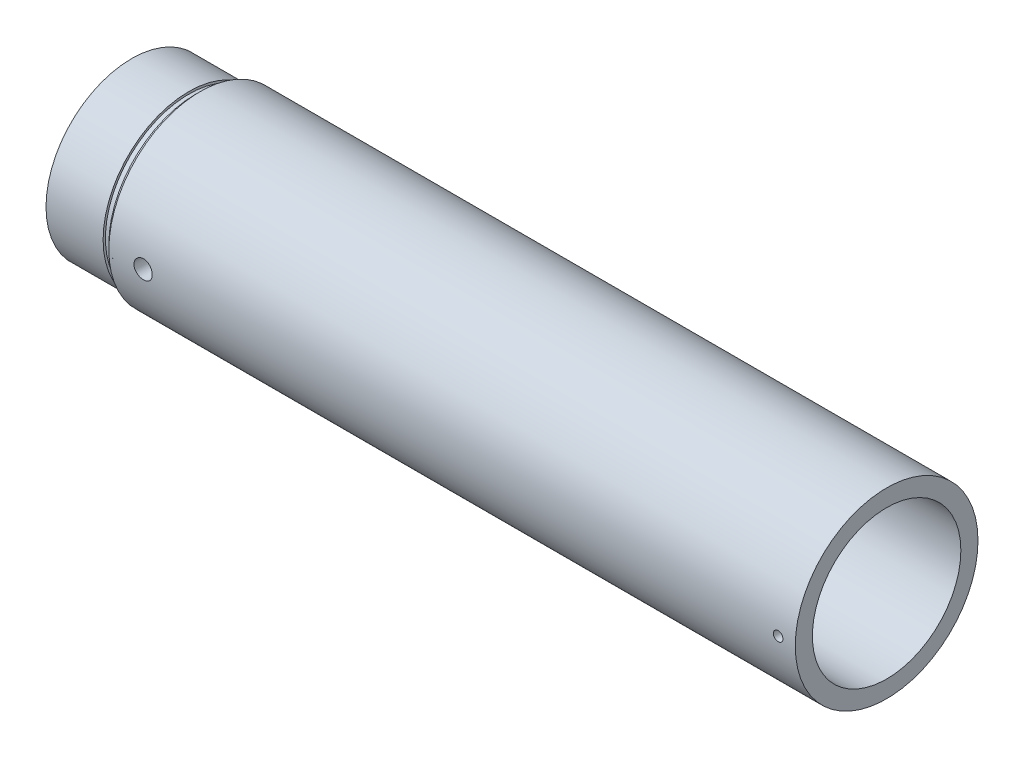
SolidWorks part; units mm, degrees
ref_plane "Front Plane" through (0, 0, 0) normal (0, 0, 1) x (1, 0, 0)
ref_plane "Top Plane" through (0, 0, 0) normal (0, 1, 0) x (1, 0, 0)
ref_plane "Right Plane" through (0, 0, 0) normal (1, 0, 0) x (0, 0, -1)
sketch "Sketch1" plane through (0, 0, 0) normal (0, 0, 1) x (1, 0, 0)
  line L0 (0, 0) -> (-259.6447, 0) construction
  line L1 (0, 0) -> (0, 37.5)
  line L2 (0, 37.5) -> (25, 37.5)
  line L3 (25, 37.5) -> (25, 36.5)
  line L4 (25, 36.5) -> (28, 36.5)
  line L5 (28, 36.5) -> (28, 38)
  line L6 (28, 38) -> (30, 38)
  line L7 (30, 38) -> (30, 40)
  line L8 (30, 40) -> (330.5, 40)
  line L9 (330.5, 40) -> (330.5, 0)
  line L10 (330.5, 0) -> (0, 0)
  dimension "D1" = 37.5
  dimension "D2" = 38
  dimension "D3" = 36.5
  dimension "D4" = 3
  dimension "D5" = 25
  dimension "D6" = 30
  dimension "D7" = 40
  dimension "D8" = 330.5
revolve "Revolve1" add sketch "Sketch1" angle 360 about L0
sketch "Sketch2" plane through (330.5, 0, 0) normal (1, 0, 0) x (0, 0, -1)
  circle A0 centre (0, 0) radius 32.5
  dimension "D1" = 65
extrude "Cut-Extrude1" cut sketch "Sketch2" against normal blind 50
cosmetic thread "Cosmetic Thread2" parameters "D2"=66
sketch "Sketch3" plane through (280.5, 0, 0) normal (1, 0, 0) x (0, 0, -1)
  circle A0 centre (0, 0) radius 30
  dimension "D1" = 60
extrude "Cut-Extrude2" cut sketch "Sketch3" against normal through all
chamfer "Chamfer1" distance 1.5 angle 45 1 edges at (280.5, 0, -32.5)
chamfer "Chamfer2" distance 1.5 angle 45 1 edges at (0, 0, -30)
sketch "Sketch4" plane through (0, 0, 0) normal (0, 0, 1) x (1, 0, 0)
  line L0 (0, 0) -> (325.6705, 0) construction
  line L1 (0, 37.5) -> (0, -37.5) construction
  circle A0 centre (45, 0) radius 4
  dimension "D1" = 8
  dimension "D2" = 45
extrude "Cut-Extrude3" cut sketch "Sketch4" against normal through all both and the other way through all
hole_wizard "M5 Tapped Hole2" positions "Sketch5" profile "Sketch7" tap size "M5" standard "GB"
sketch "Sketch5" plane through (0, 0, 0) normal (0, 0, 1) x (1, 0, 0)
  line L0 (330.5, 0) -> (30, 0) construction
  line L1 (330.5, -40) -> (330.5, 40) construction
  line L2 (30, 38) -> (30, -38) construction
  point P0 (323, 0)
  dimension "D1" = 7.5
sketch "Sketch7" plane through (323, 0, 0) normal (1, 0, 0) x (0, 1, 0)
  line L0 (0, 0) -> (0, 40)
  line L1 (0, 40) -> (2.1, 40)
  line L2 (2.1, 40) -> (2.1, 0)
  line L5 (2.1, 0) -> (0, 0)
  line L11 (0, -6.35) -> (0, 107.95) construction
  dimension "通孔螺纹孔钻头直径" = 4.2
  dimension "通孔螺纹孔钻头深度" = 40
cosmetic thread "Cosmetic thread 1" parameters "D2"=5
